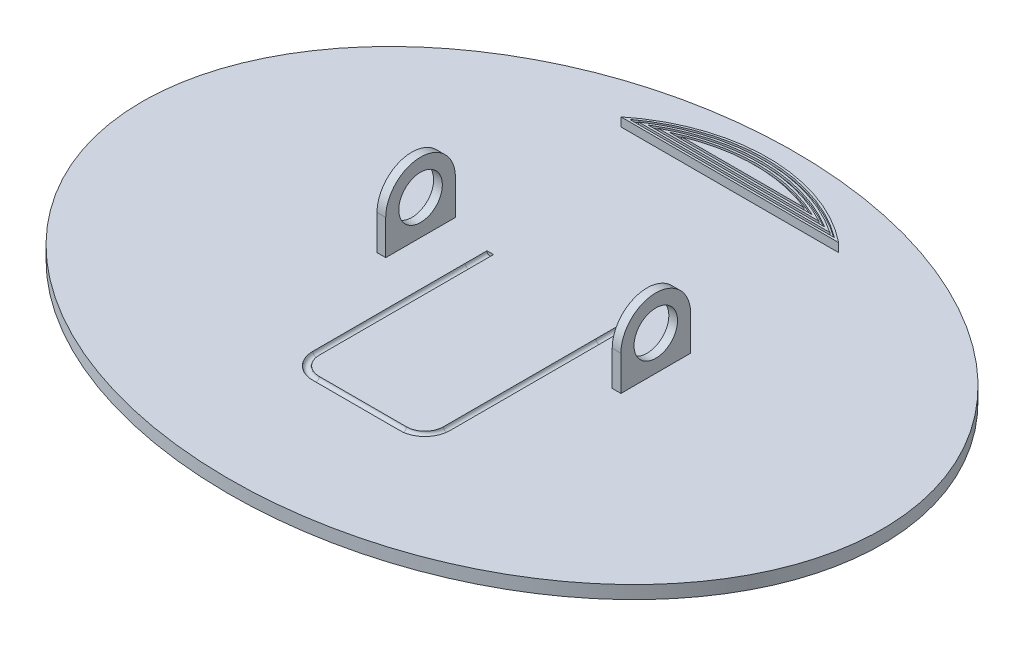
from build123d import *

# Parameters (mm, degrees)
SKETCH1_RX           = 85
SKETCH1_RY           = 65
BOSS_EXTRUDE1_DEPTH  = 3
BOSS_EXTRUDE2_START  = 28
SKETCH_2_2_R         = 5
BOSS_EXTRUDE2_DEPTH  = 2
BOSS_EXTRUDE3_START  = -26
SKETCH_2_2_2_R       = 5
BOSS_EXTRUDE3_DEPTH  = 2
CUT_SWEEP1_PROFILE_R = 0.75
BOSS_EXTRUDE4_DEPTH  = 2
CUT_EXTRUDE1_DEPTH   = 0.5
CUT_EXTRUDE2_DEPTH   = 0.5
CUT_EXTRUDE3_DEPTH   = 0.5


with BuildPart() as part:
    # Sketch1 → Boss-Extrude1 (new body)
    with BuildSketch(Plane(origin=(0, 0, 0), x_dir=(1, 0, 0), z_dir=(0, 1, 0))):
        with Locations(Location((0, 0), (0, 0, 180))):
            Ellipse(SKETCH1_RX, SKETCH1_RY)
    extrude(amount=BOSS_EXTRUDE1_DEPTH)

    # Sketch 2_2 → Boss-Extrude2 (add)
    with BuildSketch(Plane(origin=(0, 0, 0), x_dir=(0, 0, -1), z_dir=(1, 0, 0)).offset(BOSS_EXTRUDE2_START)):
        with BuildLine():
            Line((-3, 3), (-3, 11))
            ThreePointArc((-3, 11), (5, 19), (13, 11))
            Line((13, 11), (13, 3))
            Line((13, 3), (-3, 3))
        make_face()
        with Locations((5, 11)):
            Circle(SKETCH_2_2_R, mode=Mode.SUBTRACT)
    extrude(amount=-BOSS_EXTRUDE2_DEPTH)

    # Sketch 2_2 2 → Boss-Extrude3 (add)
    with BuildSketch(Plane(origin=(0, 0, 0), x_dir=(0, 0, -1), z_dir=(1, 0, 0)).offset(BOSS_EXTRUDE3_START)):
        with BuildLine():
            Line((-3, 3), (-3, 11))
            ThreePointArc((-3, 11), (5, 19), (13, 11))
            Line((13, 11), (13, 3))
            Line((13, 3), (-3, 3))
        make_face()
        with Locations((5, 11)):
            Circle(SKETCH_2_2_2_R, mode=Mode.SUBTRACT)
    extrude(amount=-BOSS_EXTRUDE3_DEPTH)

    # Cut-Sweep1: sweep along a path in Sketch3
    with BuildLine(Plane(origin=(0, 3, 0), x_dir=(1, 0, 0), z_dir=(0, 1, 0))) as cut_sweep1_path:
        Line((-15, 10), (-15, 5))
        Line((-15, 5), (-15, -30))
        ThreePointArc((-15, -30), (-13.535533906, -33.535533906), (-10, -35))
        Line((-10, -35), (10, -35))
        ThreePointArc((10, -35), (13.535533906, -33.535533906), (15, -30))
        Line((15, -30), (15, 5))
        Line((15, 5), (15, 10))
    # Cut-Sweep1 profile (on start of the path) → Cut-Sweep1 (sweep, cut)
    with BuildSketch(Plane(origin=(-15, 3, -10), x_dir=(1, 0, 0), z_dir=(0, 0, 1))):
        Circle(CUT_SWEEP1_PROFILE_R)
    sweep(path=cut_sweep1_path.line, mode=Mode.SUBTRACT)

    # Sketch23 → Boss-Extrude4 (add)
    with BuildSketch(Plane(origin=(0, 3, 0), x_dir=(1, 0, 0), z_dir=(0, 1, 0))):
        with BuildLine():
            Line((-25, 50), (25, 50))
            ThreePointArc((25, 50), (0, 58.775010008), (-25, 50))
        make_face()
    extrude(amount=BOSS_EXTRUDE4_DEPTH)

    # Sketch24 → Cut-Extrude1 (cut)
    with BuildSketch(Plane(origin=(0, 5, 0), x_dir=(1, 0, 0), z_dir=(0, 1, 0))):
        with BuildLine():
            Line((-23.532424652, 50.5), (23.532424652, 50.5))
            ThreePointArc((23.532424652, 50.5), (0, 58.275010008), (-23.532424652, 50.5))
        make_face()
        with BuildLine():
            Line((-21.967021191, 51), (21.967021191, 51))
            ThreePointArc((21.967021191, 51), (0, 57.775010008), (-21.967021191, 51))
        make_face(mode=Mode.SUBTRACT)
    extrude(amount=-CUT_EXTRUDE1_DEPTH, mode=Mode.SUBTRACT)

    # Sketch25 → Cut-Extrude2 (cut)
    with BuildSketch(Plane(origin=(0, 5, 0), x_dir=(1, 0, 0), z_dir=(0, 1, 0))):
        with BuildLine():
            Line((-20.281149623, 51.5), (20.281149623, 51.5))
            ThreePointArc((20.281149623, 51.5), (0, 57.275010008), (-20.281149623, 51.5))
        make_face()
        with BuildLine():
            Line((-18.441801431, 52), (18.441801431, 52))
            ThreePointArc((18.441801431, 52), (0, 56.775010008), (-18.441801431, 52))
        make_face(mode=Mode.SUBTRACT)
    extrude(amount=-CUT_EXTRUDE2_DEPTH, mode=Mode.SUBTRACT)

    # Sketch26 → Cut-Extrude3 (cut)
    with BuildSketch(Plane(origin=(0, 5, 0), x_dir=(1, 0, 0), z_dir=(0, 1, 0))):
        with BuildLine():
            Line((-16.397409858, 52.5), (16.397409858, 52.5))
            ThreePointArc((16.397409858, 52.5), (0, 56.275010008), (-16.397409858, 52.5))
        make_face()
        with BuildLine():
            Line((-14.058807206, 53), (14.058807206, 53))
            ThreePointArc((14.058807206, 53), (0, 55.775010008), (-14.058807206, 53))
        make_face(mode=Mode.SUBTRACT)
    extrude(amount=-CUT_EXTRUDE3_DEPTH, mode=Mode.SUBTRACT)


solid = part.part
